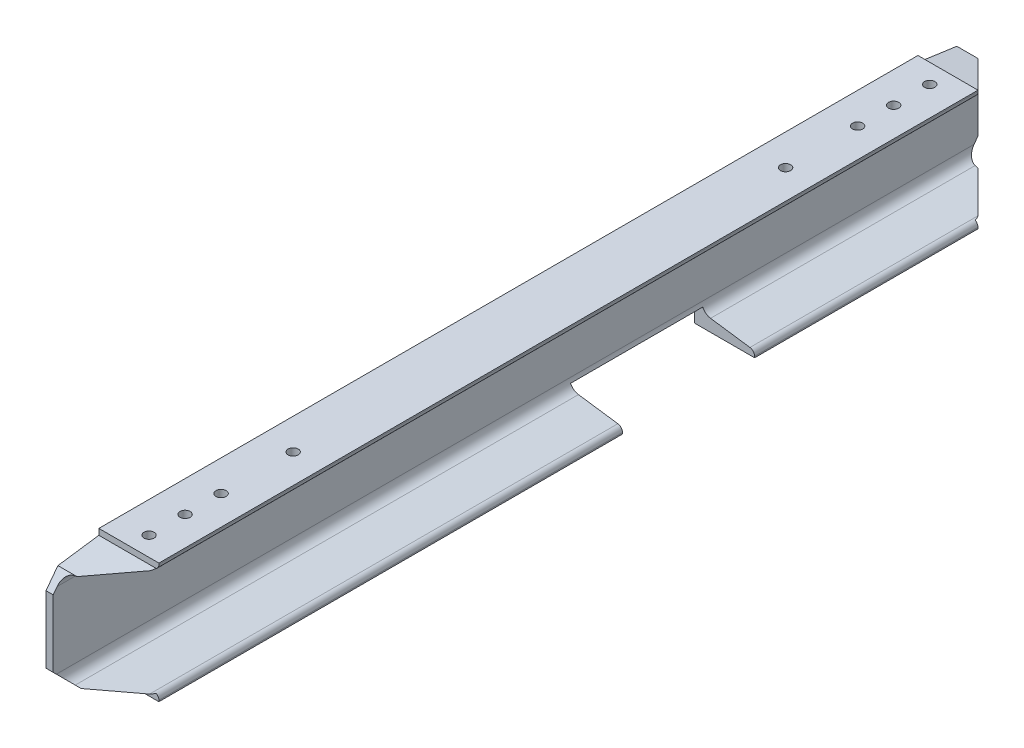
SolidWorks part; units mm, degrees
material "1023 carbon steel plate (SS)"
ref_plane "Front Plane" through (0, 0, 0) normal (0, 0, 1) x (1, 0, 0)
ref_plane "Top Plane" through (0, 0, 0) normal (0, 1, 0) x (1, 0, 0)
ref_plane "Right Plane" through (0, 0, 0) normal (1, 0, 0) x (0, 0, -1)
sketch "Sketch1" plane through (0, 0, 0) normal (0, 0, 1) x (1, 0, 0)
  line L0 (0, 0) -> (0, -100)
  line L1 (0, -100) -> (50, -100)
  line L2 (0, 0) -> (50, 0)
  line L3 (50, 0) -> (50, -1.0747)
  line L4 (50, -100) -> (50, -98.9253)
  line L5 (46.1263, -5.5309) -> (13.317, -10.1419)
  line L6 (6, -18.5592) -> (6, -81.4408)
  line L7 (13.317, -89.8581) -> (46.1263, -94.4691)
  line L8 (25, 0) -> (25, -8.5) construction
  line L9 (25, -100) -> (25, -91.5) construction
  arc A0 (6, -81.4408) -> (13.317, -89.8581) centre (14.5, -81.4408) ccw
  arc A1 (13.317, -10.1419) -> (6, -18.5592) centre (14.5, -18.5592) ccw
  arc A2 (50, -98.9253) -> (46.1263, -94.4691) centre (45.5, -98.9253) ccw
  arc A3 (50, -1.0747) -> (46.1263, -5.5309) centre (45.5, -1.0747) cw
  dimension "D8" = 8.5
  dimension "D9" = 4.5
  dimension "D1" = 100
  dimension "D2" = 50
  dimension "D3" = 50
  dimension "D4" = 6
  dimension "D5" = 8.5
  dimension "D6" = 8.5
  dimension "D7" = 98
extrude "Boss-Extrude1" add sketch "Sketch1" along normal blind 694
sketch "Sketch3" plane through (0, 0, 0) normal (-1, 0, 0) x (0, 0, 1)
  line L1 (192, -85) -> (302, -85)
  line L2 (192, -85) -> (192, -155.1716)
  line L3 (192, -155.1716) -> (302, -155.1716)
  line L4 (302, -85) -> (302, -155.1716)
  line L5 (192, -85) -> (302, -155.1716) construction
  line L6 (192, -155.1716) -> (302, -85) construction
  line L7 (694, -100) -> (0, -100) construction
  line L9 (694, 0) -> (694, -100) construction
  point P0 (247, -120.0858)
  dimension "D1" = 110
  dimension "D2" = 392
  dimension "D3" = 15
extrude "Cut-Extrude1" cut sketch "Sketch3" against normal blind 145
sketch "Sketch5" plane through (1.6557, -11.7808, 0) normal (0.1392, -0.9903, 0) x (0.9903, 0.1392, 0)
  line L0 (49.3638, 694) -> (49.3638, 0) construction
  line L2 (49.3638, 347) -> (-89.2169, 347) construction
  circle A0 centre (24.3638, 642) radius 4
  circle A1 centre (24.3638, 612) radius 4
  circle A2 centre (24.3638, 672) radius 4
  circle A3 centre (24.3638, 552) radius 4
  circle A4 centre (24.3638, 142) radius 4
  circle A5 centre (24.3638, 82) radius 4
  circle A6 centre (24.3638, 52) radius 4
  circle A7 centre (24.3638, 22) radius 4
  point P10 (49.3638, 347)
  dimension "D6" = 8
  dimension "D1" = 205
  dimension "D2" = 25
  dimension "D3" = 60
  dimension "D4" = 30
  dimension "D5" = 30
sketch "Sketch10" plane through (0, 0, 0) normal (0, 1, 0) x (1, 0, 0)
  circle A0 centre (25.7824, -22) radius 4
  circle A1 centre (25.7824, -52) radius 3.9611
  circle A2 centre (25.7824, -82) radius 4
  circle A3 centre (25.7824, -142) radius 3.9611
  circle A4 centre (25.7824, -552) radius 3.9611
  circle A5 centre (25.7824, -612) radius 3.9611
  circle A6 centre (25.7824, -642) radius 4
  circle A7 centre (25.7824, -672) radius 3.9611
hole_wizard "M10 Tapped Hole2" positions "Sketch13" profile "Sketch14" tap size "M10" standard "ISO"
sketch "Sketch13" plane through (0, 0, 0) normal (0, 1, 0) x (1, 0, 0)
  point P0 (25.7824, -142)
  point P3 (25.7824, -82)
  point P6 (25.7824, -22)
  point P9 (25.7824, -52)
  point P12 (25.7824, -552)
  point P15 (25.7824, -612)
  point P18 (25.7824, -642)
  point P21 (25.7824, -672)
sketch "Sketch14" plane through (25.7824, 0, 142) normal (1, 0, 0) x (0, 0, 1)
  line L0 (0, 0) -> (0, 27.0537)
  line L1 (0, 27.0537) -> (4.25, 24.5)
  line L2 (4.25, 24.5) -> (4.25, 0)
  line L5 (4.25, 0) -> (0, 0)
  line L10 (0, 27.0537) -> (-4.25, 24.5) construction
  line L11 (0, -6.35) -> (0, 107.95) construction
  dimension "螺纹孔钻头直径" = 8.5
  dimension "螺纹孔钻头深度" = 24.5
  dimension "导头角度" = 118
cosmetic thread "Cosmetic thread 9" parameters "D1"=20, "D2"=10
cosmetic thread "Cosmetic thread 10" parameters "D1"=20, "D2"=10
cosmetic thread "Cosmetic thread 11" parameters "D1"=20, "D2"=10
cosmetic thread "Cosmetic thread 12" parameters "D1"=20, "D2"=10
cosmetic thread "Cosmetic thread 13" parameters "D1"=20, "D2"=10
cosmetic thread "Cosmetic thread 14" parameters "D1"=20, "D2"=10
cosmetic thread "Cosmetic thread 15" parameters "D1"=20, "D2"=10
cosmetic thread "Cosmetic thread 16" parameters "D1"=20, "D2"=10
sketch "Sketch15" plane through (0, 0, 0) normal (0, 0, -1) x (-1, 0, 0)
  line L8 (0, 0) -> (-50, 0)
  line L9 (-50, 0) -> (-50, -1.0747)
  line L10 (-46.1263, -5.5309) -> (-13.317, -10.1419)
  line L11 (-6, -18.5592) -> (-6, -81.4408)
  line L12 (-13.317, -89.8581) -> (-46.1263, -94.4691)
  line L13 (-50, -98.9253) -> (-50, -100)
  line L14 (-50, -100) -> (0, -100)
  line L15 (0, -100) -> (0, 0)
  line L16 (0, 0) -> (-50, 0)
  line L17 (-50, 0) -> (-50, -1.0747)
  line L18 (-46.1263, -5.5309) -> (-13.317, -10.1419)
  line L19 (-6, -18.5592) -> (-6, -81.4408)
  line L20 (-13.317, -89.8581) -> (-46.1263, -94.4691)
  line L21 (-50, -98.9253) -> (-50, -100)
  line L22 (-50, -100) -> (0, -100)
  line L23 (0, -100) -> (0, 0)
  arc A4 (-50, -1.0747) -> (-46.1263, -5.5309) centre (-45.5, -1.0747) ccw
  arc A5 (-6, -18.5592) -> (-13.317, -10.1419) centre (-14.5, -18.5592) ccw
  arc A6 (-13.317, -89.8581) -> (-6, -81.4408) centre (-14.5, -81.4408) ccw
  arc A7 (-46.1263, -94.4691) -> (-50, -98.9253) centre (-45.5, -98.9253) ccw
  arc A8 (-50, -1.0747) -> (-46.1263, -5.5309) centre (-45.5, -1.0747) ccw
  arc A9 (-6, -18.5592) -> (-13.317, -10.1419) centre (-14.5, -18.5592) ccw
  arc A10 (-13.317, -89.8581) -> (-6, -81.4408) centre (-14.5, -81.4408) ccw
  arc A11 (-46.1263, -94.4691) -> (-50, -98.9253) centre (-45.5, -98.9253) ccw
  dimension "D1" = 0
extrude "Boss-Extrude2" add sketch "Sketch15" along normal blind 44
sketch "Sketch17" plane through (0, 0, 694) normal (0, 0, 1) x (1, 0, 0)
  line L8 (50, 0) -> (0, 0)
  line L9 (0, 0) -> (0, -100)
  line L10 (0, -100) -> (50, -100)
  line L11 (50, -100) -> (50, -98.9253)
  line L12 (46.1263, -94.4691) -> (13.317, -89.8581)
  line L13 (6, -81.4408) -> (6, -18.5592)
  line L14 (13.317, -10.1419) -> (46.1263, -5.5309)
  line L15 (50, -1.0747) -> (50, 0)
  line L16 (50, 0) -> (0, 0)
  line L17 (0, 0) -> (0, -100)
  line L18 (0, -100) -> (50, -100)
  line L19 (50, -100) -> (50, -98.9253)
  line L20 (46.1263, -94.4691) -> (13.317, -89.8581)
  line L21 (6, -81.4408) -> (6, -18.5592)
  line L22 (13.317, -10.1419) -> (46.1263, -5.5309)
  line L23 (50, -1.0747) -> (50, 0)
  arc A4 (50, -98.9253) -> (46.1263, -94.4691) centre (45.5, -98.9253) ccw
  arc A5 (6, -81.4408) -> (13.317, -89.8581) centre (14.5, -81.4408) ccw
  arc A6 (13.317, -10.1419) -> (6, -18.5592) centre (14.5, -18.5592) ccw
  arc A7 (46.1263, -5.5309) -> (50, -1.0747) centre (45.5, -1.0747) ccw
  arc A8 (50, -98.9253) -> (46.1263, -94.4691) centre (45.5, -98.9253) ccw
  arc A9 (6, -81.4408) -> (13.317, -89.8581) centre (14.5, -81.4408) ccw
  arc A10 (13.317, -10.1419) -> (6, -18.5592) centre (14.5, -18.5592) ccw
  arc A11 (46.1263, -5.5309) -> (50, -1.0747) centre (45.5, -1.0747) ccw
  dimension "D1" = 0
extrude "Boss-Extrude3" add sketch "Sketch17" along normal blind 44
sketch "Sketch16" plane through (0, 0, 0) normal (-1, 0, 0) x (0, 0, 1)
  line L0 (6, -100) -> (-44, -100)
  line L1 (192, -100) -> (-44, -100) construction
  line L2 (-44, -100) -> (-44, 0)
  line L3 (-44, 0) -> (6, 0)
  line L4 (738, 0) -> (-44, 0) construction
  line L5 (6, 0) -> (6, -4.9865)
  line L6 (6, -4.9865) -> (-38, -11.1703)
  line L7 (-38, -11.1703) -> (-38, -88.8297)
  line L8 (-38, -88.8297) -> (6, -95.0135)
  line L9 (6, -95.0135) -> (6, -100)
  line L10 (-19, -100) -> (-19, -91.5) construction
  line L11 (347, 0) -> (347, -169.6383) construction
  line L12 (738, 0) -> (-44, 0) construction
  line L13 (713, -100) -> (713, -91.5) construction
  line L14 (688, -95.0135) -> (688, -100)
  line L15 (732, -88.8297) -> (688, -95.0135)
  line L16 (732, -11.1703) -> (732, -88.8297)
  line L17 (688, -4.9865) -> (732, -11.1703)
  line L18 (688, 0) -> (688, -4.9865)
  line L19 (738, 0) -> (688, 0)
  line L20 (738, -100) -> (738, 0)
  line L21 (688, -100) -> (738, -100)
  dimension "D1" = 50
  dimension "D2" = 50
  dimension "D3" = 6
  dimension "D4" = 25
  dimension "D5" = 8.5
  dimension "D6" = 8
  dimension "D7" = 8
extrude "Cut-Extrude3" cut sketch "Sketch16" against normal blind 100
chamfer "Chamfer1" distance 10 angle 45 4 edges at (5.1492, -11.1703, 732) (5.1492, -88.8297, 732) (5.1492, -11.1703, -38) (5.1492, -88.8297, -38)
sketch "Sketch18" plane through (0, 0, 0) normal (-1, 0, 0) x (0, 0, 1)
  line L0 (688, 0) -> (6, 0) construction
  circle A0 centre (334.5, -20) radius 7.5283
  circle A1 centre (359.5, -20) radius 7.5283
  point P6 (347, 0)
  dimension "D1" = 25
  dimension "D2" = 20
  dimension "D3" = 12.5
hole_wizard "M6 Tapped Hole1" positions "Sketch19" profile "Sketch20" tap size "M6" standard "ISO"
sketch "Sketch19" plane through (0, 0, 0) normal (-1, 0, 0) x (0, 0, 1)
  point P0 (334.5, -20)
  point P3 (359.5, -20)
sketch "Sketch20" plane through (0, -20, 334.5) normal (0, 1, 0) x (0, 0, 1)
  line L0 (0, 0) -> (0, 16.5022)
  line L1 (0, 16.5022) -> (2.5, 15)
  line L2 (2.5, 15) -> (2.5, 0)
  line L5 (2.5, 0) -> (0, 0)
  line L10 (0, 16.5022) -> (-2.5, 15) construction
  line L11 (0, -6.35) -> (0, 107.95) construction
  dimension "螺纹孔钻头直径" = 5
  dimension "螺纹孔钻头深度" = 15
  dimension "导头角度" = 118
cosmetic thread "Cosmetic thread 17" parameters "D1"=12, "D2"=6
cosmetic thread "Cosmetic thread 18" parameters "D1"=12, "D2"=6
